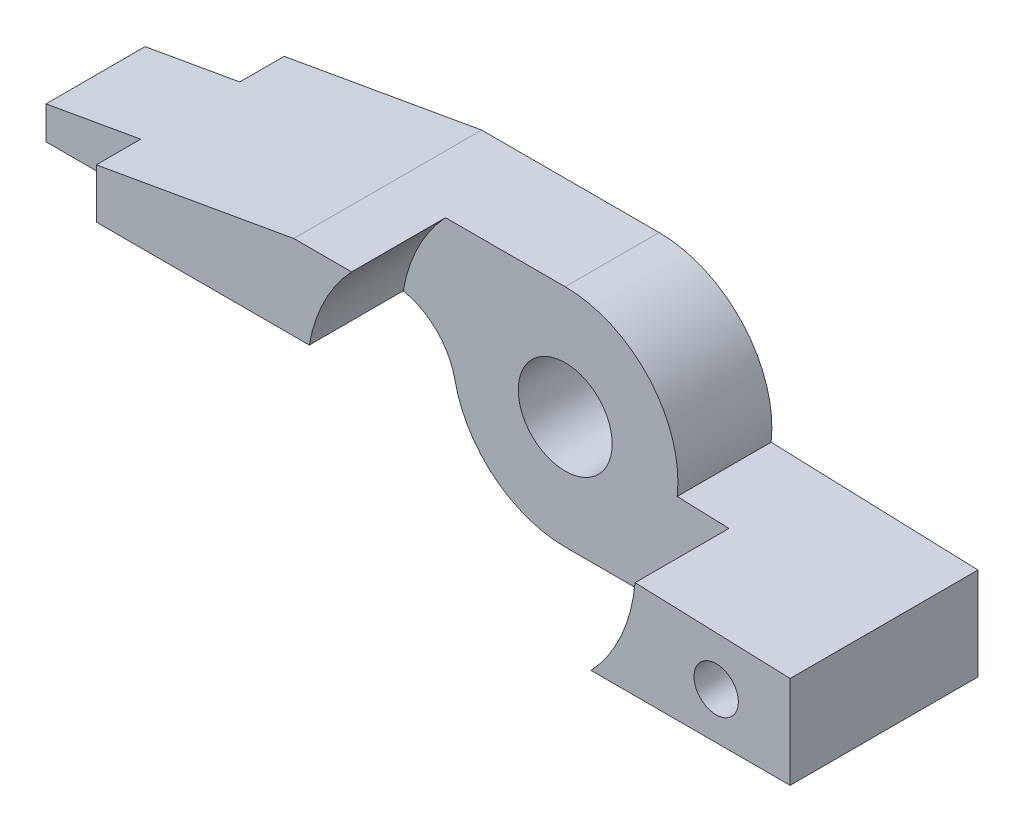
from build123d import *

# Parameters (mm, degrees)
SKETCH1_R           = 6.35
BOSS_EXTRUDE1_DEPTH = 25.4
SKETCH2_R           = 22.23
CUT_EXTRUDE1_DEPTH  = 12.7
CUT_EXTRUDE_1_REACH = 169.736
SCALE_1_SCALE       = 0.5
SCALE_2_SCALE       = 0.5
SKETCH_2_R          = 0.75
CUT_EXTRUDE_2_DEPTH = 18.517255065
SKETCH_3_W          = 3.175
SKETCH_3_H          = 0.9525
CUT_EXTRUDE_3_DEPTH = 6.35
CUT_EXTRUDE_4_DEPTH = 1.5
CUT_EXTRUDE_5_DEPTH = 1.5


with BuildPart() as part:
    # Sketch1 → Boss-Extrude1 (new body)
    with BuildSketch(Plane.XY):
        with BuildLine():
            Line((0, -15.24), (165.1, -15.24))
            Line((165.1, -15.24), (165.1, -6.98))
            Line((165.1, -6.98), (27.790517271, -2.185047205))
            Line((27.790517271, -2.185047205), (22.140950977, -1.987760002))
            Line((22.140950977, -1.987760002), (15.139966118, -1.743280224))
            ThreePointArc((15.139966118, -1.743280224), (11.375965687, 10.14125262), (0, 15.24))
            Line((0, 15.24), (-24, 15.24))
            Line((-24, 15.24), (-63.5, 8.26))
            Line((-63.5, 8.26), (-63.5, 0))
            Line((-63.5, 0), (-50.8, 0))
            Line((-50.8, 0), (-50.8, 3.81))
            Line((-50.8, 3.81), (-46.99, 3.81))
            Line((-46.99, 3.81), (-21.901068467, 3.81))
            ThreePointArc((-21.901068467, 3.81), (-17.369676473, 1.405708043), (-14.920995783, -3.10185184))
            ThreePointArc((-14.920995783, -3.10185184), (-9.617311942, -11.82222107), (0, -15.24))
        make_face()
        Circle(SKETCH1_R, mode=Mode.SUBTRACT)
    extrude(amount=BOSS_EXTRUDE1_DEPTH)

    # Sketch2 → Cut-Extrude1 (cut)
    with BuildSketch(Plane.XY.offset(25.4)):
        Circle(SKETCH2_R)
    extrude(amount=-CUT_EXTRUDE1_DEPTH, mode=Mode.SUBTRACT)

    # 草图1 → 切除-拉伸1 (cut, up to next)
    with BuildSketch(Plane.XY.offset(25.4), mode=Mode.PRIVATE) as cut_extrude_1_sk1:
        Polygon((43.109053356, -15.24), (43.109053356, -2.719982272), (165.1, -6.98), (165.1, -15.24), align=None)
    cut_extrude_1_tool1 = extrude(cut_extrude_1_sk1.sketch, amount=-CUT_EXTRUDE_1_REACH, mode=Mode.PRIVATE) & part.part
    add(cut_extrude_1_tool1.solids().sort_by_distance((99.936391, -9.972218, 25.4))[0], mode=Mode.SUBTRACT)


with BuildPart() as part_1:
    # 缩放比例1: scaled about (0, 0, 0)
    add(part.part.scale(SCALE_1_SCALE))


with BuildPart() as part_2:
    # 缩放比例2: scaled about (0, 0, 0)
    add(part_1.part.scale(SCALE_2_SCALE))

    # 草图2 → 切除-拉伸2 (cut, through all)
    with BuildSketch(Plane.XY.offset(6.35)):
        with Locations((8.277263339, -2.244997784)):
            Circle(SKETCH_2_R)
    extrude(amount=-CUT_EXTRUDE_2_DEPTH, mode=Mode.SUBTRACT)

    # 草图3 → 切除-拉伸3 (cut)
    with BuildSketch(Plane.XY.offset(6.35)):
        with Locations((-14.2875, 0.47625)):
            Rectangle(SKETCH_3_W, SKETCH_3_H)
    extrude(amount=-CUT_EXTRUDE_3_DEPTH, mode=Mode.SUBTRACT)

    # 草图4 → 切除-拉伸4 (cut)
    with BuildSketch(Plane.XY.offset(6.35)):
        Polygon((-15.875, 2.065), (-15.875, 0.9525), (-12.675, 0.9525), (-12.675, 2.630468354), align=None)
    extrude(amount=-CUT_EXTRUDE_4_DEPTH, mode=Mode.SUBTRACT)

    # 草图5 → 切除-拉伸5 (cut)
    with BuildSketch(Plane(origin=(0, 0, 0), x_dir=(-1, 0, 0), z_dir=(0, 0, -1))):
        Polygon((15.875, 2.065), (15.875, 0.9525), (12.675, 0.9525), (12.675, 2.630468354), align=None)
    extrude(amount=-CUT_EXTRUDE_5_DEPTH, mode=Mode.SUBTRACT)


solid = part_2.part
